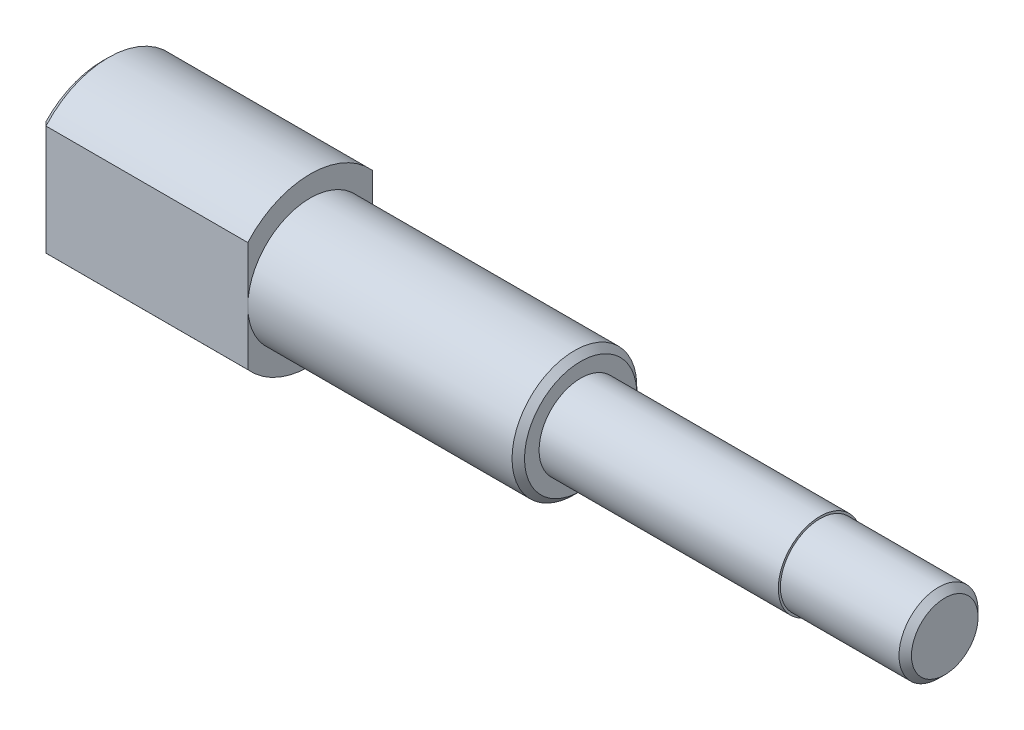
SolidWorks part; units mm, degrees
material "304"
ref_plane "Front Plane" through (0, 0, 0) normal (0, 0, 1) x (1, 0, 0)
ref_plane "Top Plane" through (0, 0, 0) normal (0, 1, 0) x (1, 0, 0)
ref_plane "Right Plane" through (0, 0, 0) normal (1, 0, 0) x (0, 0, -1)
sketch "Sketch1" plane through (0, 0, 0) normal (0, 0, 1) x (1, 0, 0)
  line L0 (0, 0) -> (40.5, 0) construction
  line L2 (0, 0) -> (40.5, 0)
  line L4 (23, 2) -> (34.5, 2)
  line L6 (10, 3) -> (23, 3)
  line L7 (23, 3) -> (23, 2)
  line L8 (0, 0) -> (0, 4)
  line L9 (0, 4) -> (10, 4)
  line L10 (10, 4) -> (10, 3)
  line L11 (34.5, 2) -> (34.5, 1.9)
  line L12 (34.5, 1.9) -> (40.5, 1.9)
  line L13 (40.5, 1.9) -> (40.5, 0)
  dimension "D1" = 2
  dimension "D2" = 11.5
  dimension "D3" = 10
  dimension "D4" = 3
  dimension "D5" = 4
  dimension "D6" = 23
  dimension "D7" = 6
  dimension "D8" = 1.9
revolve "Revolve1" add sketch "Sketch1" angle 360 about L0
sketch "Sketch2" plane through (0, 0, 0) normal (-1, 0, 0) x (0, 0, 1)
  line L0 (0, 0) -> (0, 4.5687) construction
  line L5 (-4, 4.6507) -> (-3, 4.6507)
  line L6 (-4, 4.6507) -> (-4, -4.6507)
  line L7 (-4, -4.6507) -> (-3, -4.6507)
  line L8 (-3, 4.6507) -> (-3, -4.6507)
  line L9 (3, 4.254) -> (4, 4.254)
  line L10 (3, 4.254) -> (3, -4.254)
  line L11 (3, -4.254) -> (4, -4.254)
  line L12 (4, 4.254) -> (4, -4.254)
  point P15 (-4, 0)
  point P16 (4, 0)
  dimension "D1" = 3
  dimension "D2" = 3
  dimension "D3" = 4
  dimension "D4" = 4
extrude "Cut-Extrude1" cut sketch "Sketch2" against normal up to next
chamfer "Chamfer2" distance 0.3 angle 45 6 edges at (0, 0, 3) (0, 4, 0) (0, -4, 0) (0, 0, -3) (23, 0, 3) (40.5, 0, 1.9)
